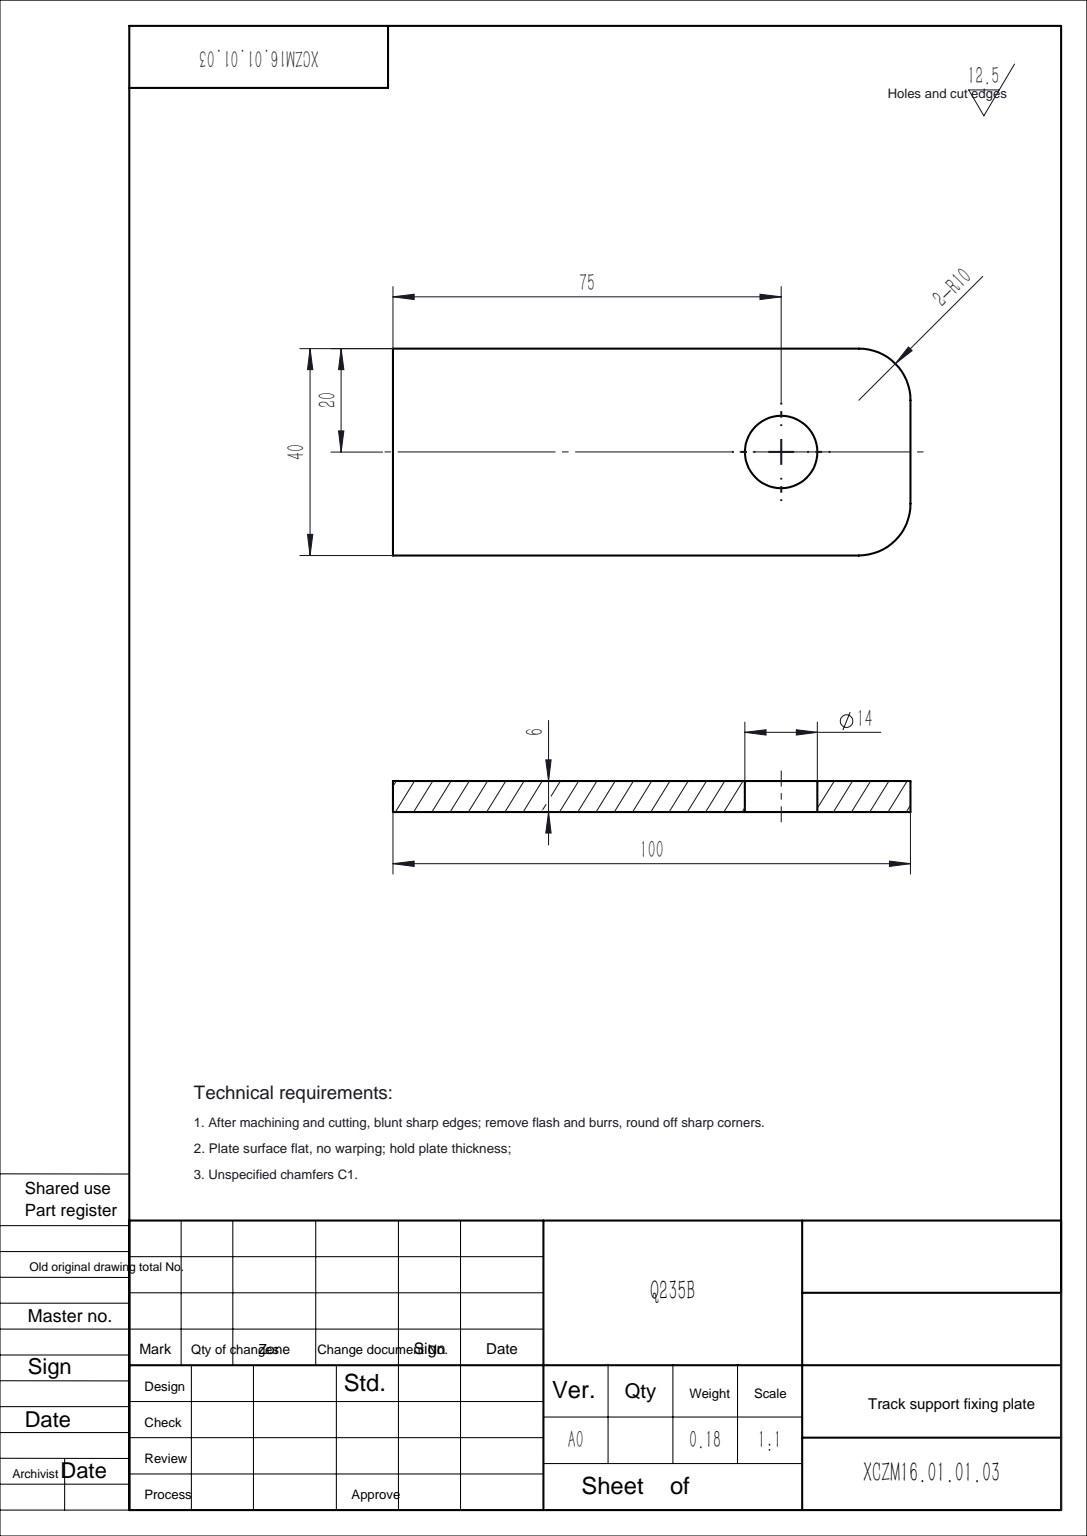
from build123d import *

# Parameters (mm, degrees)
SKETCH1_R           = 7
BOSS_EXTRUDE1_DEPTH = 6


with BuildPart() as part:
    # Sketch1 → Boss-Extrude1 (new body)
    with BuildSketch(Plane(origin=(0, 0, 0), x_dir=(1, 0, 0), z_dir=(0, 1, 0))):
        with BuildLine():
            Line((40, -20), (-50, -20))
            Line((-50, -20), (-50, 20))
            Line((-50, 20), (40, 20))
            ThreePointArc((40, 20), (47.071067812, 17.071067812), (50, 10))
            Line((50, 10), (50, -10))
            ThreePointArc((50, -10), (47.071067812, -17.071067812), (40, -20))
        make_face()
        with Locations(Location((25, 0, 0), (0, 0, 270))):
            Circle(SKETCH1_R, mode=Mode.SUBTRACT)
    extrude(amount=BOSS_EXTRUDE1_DEPTH)


solid = part.part
